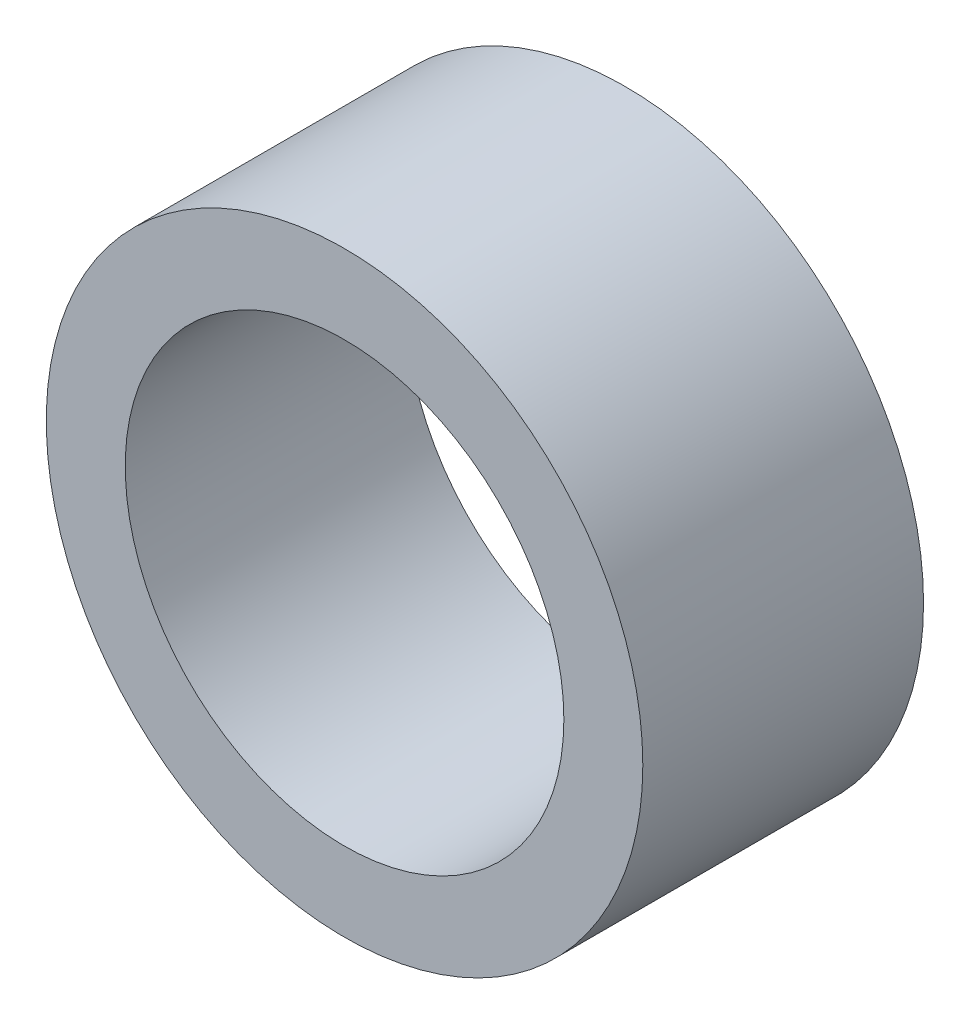
from build123d import *

# Parameters (mm, degrees)
SKETCH1_R           = 8.5
SKETCH1_R_2         = 6.25
BOSS_EXTRUDE1_DEPTH = 8


with BuildPart() as part:
    # Sketch1 → Boss-Extrude1 (new body)
    with BuildSketch(Plane.XY):
        Circle(SKETCH1_R)
        Circle(SKETCH1_R_2, mode=Mode.SUBTRACT)
    extrude(amount=BOSS_EXTRUDE1_DEPTH)


solid = part.part
